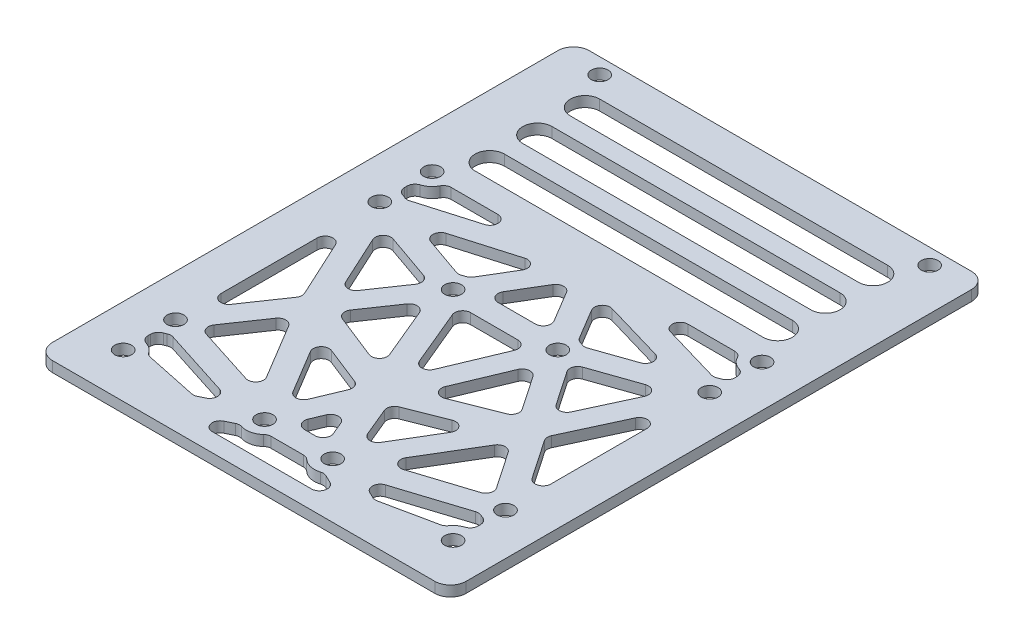
from build123d import *

# Parameters (mm, degrees)
SKETCH1_W              = 79
SKETCH1_H              = 102.5
SKETCH1_R              = 1.6
BOSS_EXTRUDE1_DEPTH    = 2
CUT_EXTRUDE1_DEPTH     = 69.558369292
R1_5_CUTOUT_FILLET_R   = 1.5
R3_OUTER_EDGE_FILLET_R = 3


with BuildPart() as part:
    # Sketch1 → Boss-Extrude1 (new body)
    with BuildSketch(Plane(origin=(0, 0, 0), x_dir=(1, 0, 0), z_dir=(0, 1, 0))):
        with Locations((0, 4.75)):
            Rectangle(SKETCH1_W, SKETCH1_H)
        with Locations(Location((-31.5, 11, 0), (0, 0, 270))):
            Circle(SKETCH1_R, mode=Mode.SUBTRACT)
        with Locations(Location((-31.5, 21, 0), (0, 0, 270))):
            Circle(SKETCH1_R, mode=Mode.SUBTRACT)
        with Locations(Location((31.5, 11, 0), (0, 0, 90))):
            Circle(SKETCH1_R, mode=Mode.SUBTRACT)
        with Locations(Location((31.5, 21, 0), (0, 0, 90))):
            Circle(SKETCH1_R, mode=Mode.SUBTRACT)
        with Locations(Location((-6.5, -36, 0), (0, 0, 270))):
            Circle(SKETCH1_R, mode=Mode.SUBTRACT)
        with Locations(Location((6.5, -36, 0), (0, 0, 90))):
            Circle(SKETCH1_R, mode=Mode.SUBTRACT)
        with Locations(Location((-10, 3.5, 0), (0, 0, 270))):
            Circle(SKETCH1_R, mode=Mode.SUBTRACT)
        with Locations(Location((10, 3.5, 0), (0, 0, 90))):
            Circle(SKETCH1_R, mode=Mode.SUBTRACT)
        with Locations(Location((-31.5, 53, 0), (0, 0, 270))):
            Circle(SKETCH1_R, mode=Mode.SUBTRACT)
        with Locations(Location((31.5, 53, 0), (0, 0, 90))):
            Circle(SKETCH1_R, mode=Mode.SUBTRACT)
        with Locations(Location((-31.5, -28, 0), (0, 0, 270))):
            Circle(SKETCH1_R, mode=Mode.SUBTRACT)
        with Locations(Location((-31.5, -38, 0), (0, 0, 270))):
            Circle(SKETCH1_R, mode=Mode.SUBTRACT)
        with Locations(Location((31.5, -38, 0), (0, 0, 90))):
            Circle(SKETCH1_R, mode=Mode.SUBTRACT)
        with Locations(Location((31.5, -28, 0), (0, 0, 90))):
            Circle(SKETCH1_R, mode=Mode.SUBTRACT)
    extrude(amount=BOSS_EXTRUDE1_DEPTH)

    # Sketch2 → Cut-Extrude1 (cut, through all)
    with BuildSketch(Plane(origin=(0, 2, 0), x_dir=(1, 0, 0), z_dir=(0, 1, 0))):
        with BuildLine():
            Line((-27.5, 43.4), (27.5, 43.4))
            ThreePointArc((27.5, 43.4), (30.3, 46.2), (27.5, 49))
            Line((27.5, 49), (-27.5, 49))
            ThreePointArc((-27.5, 49), (-30.3, 46.2), (-27.5, 43.4))
        make_face()
        with BuildLine():
            Line((-27.5, 34.3), (27.5, 34.3))
            ThreePointArc((27.5, 34.3), (30.3, 37.1), (27.5, 39.9))
            Line((27.5, 39.9), (-27.5, 39.9))
            ThreePointArc((-27.5, 39.9), (-30.3, 37.1), (-27.5, 34.3))
        make_face()
        with BuildLine():
            Line((-27.5, 25.2), (27.5, 25.2))
            ThreePointArc((27.5, 25.2), (30.3, 28), (27.5, 30.8))
            Line((27.5, 30.8), (-27.5, 30.8))
            ThreePointArc((-27.5, 30.8), (-30.3, 28), (-27.5, 25.2))
        make_face()
        with BuildLine():
            Line((-31.5, 17.5), (-31.5, 14.5))
            ThreePointArc((-31.5, 14.5), (-30.423705251, 14.330403821), (-29.451716488, 13.838051207))
            Line((-29.451716488, 13.838051207), (-7.668957034, 20.2))
            Line((-7.668957034, 20.2), (-28.092654993, 20.2))
            ThreePointArc((-28.092654993, 20.2), (-29.326293488, 18.256826655), (-31.5, 17.5))
        make_face()
        with BuildLine():
            ThreePointArc((29.451716488, 13.838051207), (30.423705251, 14.330403821), (31.5, 14.5))
            Line((31.5, 14.5), (31.5, 17.5))
            ThreePointArc((31.5, 17.5), (29.326293488, 18.256826655), (28.092654993, 20.2))
            Line((28.092654993, 20.2), (7.668957034, 20.2))
            Line((7.668957034, 20.2), (29.451716488, 13.838051207))
        make_face()
        with BuildLine():
            Line((-24.452290628, 10.818556238), (-11.899535217, 6.439688072))
            ThreePointArc((-11.899535217, 6.439688072), (-11.192938065, 6.790425318), (-10.425740034, 6.974009992))
            Line((-10.425740034, 6.974009992), (-4.662637344, 16.598391483))
            Line((-4.662637344, 16.598391483), (-24.452290628, 10.818556238))
        make_face()
        Polygon((-6.206589312, 5.65), (6.206589312, 5.65), (0, 16.015004152), align=None)
        with BuildLine():
            Line((11.899535217, 6.439688072), (24.452290628, 10.818556238))
            Line((24.452290628, 10.818556238), (4.662637344, 16.598391483))
            Line((4.662637344, 16.598391483), (10.425740034, 6.974009992))
            ThreePointArc((10.425740034, 6.974009992), (11.192938065, 6.790425318), (11.899535217, 6.439688072))
        make_face()
        Polygon((-27.420486956, 7.299854547), (-20.389131694, -7.907495205), (-13.357776432, 2.394257853), align=None)
        Polygon((-17.456513392, -11.238449922), (-3.946122396, -16.570590362), (-10.457154201, -0.983574828), align=None)
        Polygon((-6.771858845, 1.35), (0, -14.86141966), (6.771858845, 1.35), align=None)
        Polygon((-31.5, 5.87701259), (-31.5, -24.186209235), (-23.213342702, -12.045292729), align=None)
        Polygon((13.357776432, 2.394257853), (20.389131694, -7.907495205), (27.420486956, 7.299854547), align=None)
        Polygon((10.457154201, -0.983574828), (3.946122396, -16.570590362), (17.456513392, -11.238449922), align=None)
        Polygon((23.213342702, -12.045292729), (31.5, -24.186209235), (31.5, 5.87701259), align=None)
        Polygon((-28.098995565, -26.830923802), (-11.279390947, -32.21319728), (-20.866565579, -16.234572893), align=None)
        Polygon((-15.647599969, -16.575151194), (-6.844560738, -31.246883245), (-2.829139335, -21.634207764), align=None)
        Polygon((-3.271858845, -33.85), (3.271858845, -33.85), (0, -26.017368219), align=None)
        Polygon((2.829139335, -21.634207764), (6.844560738, -31.246883245), (15.647599969, -16.575151194), align=None)
        Polygon((20.866565579, -16.234572893), (11.279390947, -32.21319728), (28.098995565, -26.830923802), align=None)
        with BuildLine():
            Line((-28.354506597, -36.465115232), (-17.21554823, -38.810303281))
            Line((-17.21554823, -38.810303281), (-12.270862978, -36.410721464))
            Line((-12.270862978, -36.410721464), (-29.52486957, -30.889439354))
            ThreePointArc((-29.52486957, -30.889439354), (-30.466326391, -31.343877819), (-31.5, -31.5))
            Line((-31.5, -31.5), (-31.5, -34.5))
            ThreePointArc((-31.5, -34.5), (-29.645558937, -35.031658991), (-28.354506597, -36.465115232))
        make_face()
        with BuildLine():
            Line((-8.046002547, -39.140043969), (-16, -43))
            Line((-16, -43), (16, -43))
            Line((16, -43), (8.046002547, -39.140043969))
            ThreePointArc((8.046002547, -39.140043969), (5.716046361, -39.41107266), (3.738207104, -38.15))
            Line((3.738207104, -38.15), (-3.738207104, -38.15))
            ThreePointArc((-3.738207104, -38.15), (-5.716046361, -39.41107266), (-8.046002547, -39.140043969))
        make_face()
        with BuildLine():
            Line((12.270862978, -36.410721464), (17.21554823, -38.810303281))
            Line((17.21554823, -38.810303281), (28.354506597, -36.465115232))
            ThreePointArc((28.354506597, -36.465115232), (29.645558937, -35.031658991), (31.5, -34.5))
            Line((31.5, -34.5), (31.5, -31.5))
            ThreePointArc((31.5, -31.5), (30.466326391, -31.343877819), (29.52486957, -30.889439354))
            Line((29.52486957, -30.889439354), (12.270862978, -36.410721464))
        make_face()
    extrude(amount=-CUT_EXTRUDE1_DEPTH, mode=Mode.SUBTRACT)

    # R1.5 cutout fillet
    r1_5_cutout_fillet_edges = [part.edges().sort_by_distance(p)[0] for p in [
        (-28.354506597, 1, 36.465115232),
        (-31.5, 1, 34.5),
        (-31.5, 1, 31.5),
        (-29.52486957, 1, 30.889439354),
        (-12.270862978, 1, 36.410721464),
        (-17.21554823, 1, 38.810303281),
        (28.098995565, 1, 26.830923802),
        (11.279390947, 1, 32.21319728),
        (20.866565579, 1, 16.234572893),
        (-3.271858845, 1, 33.85),
        (0, 1, 26.017368219),
        (3.271858845, 1, 33.85),
        (15.647599969, 1, 16.575151194),
        (6.844560738, 1, 31.246883245),
        (2.829139335, 1, 21.634207764),
        (28.354506597, 1, 36.465115232),
        (17.21554823, 1, 38.810303281),
        (12.270862978, 1, 36.410721464),
        (29.52486957, 1, 30.889439354),
        (31.5, 1, 31.5),
        (31.5, 1, 34.5),
        (8.046002547, 1, 39.140043969),
        (16, 1, 43),
        (-16, 1, 43),
        (-8.046002547, 1, 39.140043969),
        (-3.738207104, 1, 38.15),
        (3.738207104, 1, 38.15),
        (6.206589312, 1, -5.65),
        (-6.206589312, 1, -5.65),
        (0, 1, -16.015004152),
        (-10.425740034, 1, -6.974009992),
        (-11.899535217, 1, -6.439688072),
        (-24.452290628, 1, -10.818556238),
        (-4.662637344, 1, -16.598391483),
        (10.425740034, 1, -6.974009992),
        (4.662637344, 1, -16.598391483),
        (24.452290628, 1, -10.818556238),
        (11.899535217, 1, -6.439688072),
        (-27.420486956, 1, -7.299854547),
        (-13.357776432, 1, -2.394257853),
        (-20.389131694, 1, 7.907495205),
        (28.092654993, 1, -20.2),
        (31.5, 1, -17.5),
        (31.5, 1, -14.5),
        (29.451716488, 1, -13.838051207),
        (7.668957034, 1, -20.2),
        (-31.5, 1, -17.5),
        (-28.092654993, 1, -20.2),
        (-7.668957034, 1, -20.2),
        (-29.451716488, 1, -13.838051207),
        (-31.5, 1, -14.5),
        (-20.866565579, 1, 16.234572893),
        (-11.279390947, 1, 32.21319728),
        (-28.098995565, 1, 26.830923802),
        (-15.647599969, 1, 16.575151194),
        (-2.829139335, 1, 21.634207764),
        (-6.844560738, 1, 31.246883245),
        (31.5, 1, -5.87701259),
        (31.5, 1, 24.186209235),
        (23.213342702, 1, 12.045292729),
        (17.456513392, 1, 11.238449922),
        (3.946122396, 1, 16.570590362),
        (10.457154201, 1, 0.983574828),
        (0, 1, 14.86141966),
        (-6.771858845, 1, -1.35),
        (6.771858845, 1, -1.35),
        (-17.456513392, 1, 11.238449922),
        (-10.457154201, 1, 0.983574828),
        (-3.946122396, 1, 16.570590362),
        (-31.5, 1, -5.87701259),
        (-23.213342702, 1, 12.045292729),
        (-31.5, 1, 24.186209235),
        (27.420486956, 1, -7.299854547),
        (20.389131694, 1, 7.907495205),
        (13.357776432, 1, -2.394257853),
    ]]
    fillet(r1_5_cutout_fillet_edges, radius=R1_5_CUTOUT_FILLET_R)

    # R3 outer edge fillet
    r3_outer_edge_fillet_edges = [part.edges().sort_by_distance(p)[0] for p in [
        (-39.5, 1, -56),
        (39.5, 1, -56),
        (39.5, 1, 46.5),
        (-39.5, 1, 46.5),
    ]]
    fillet(r3_outer_edge_fillet_edges, radius=R3_OUTER_EDGE_FILLET_R)


solid = part.part
